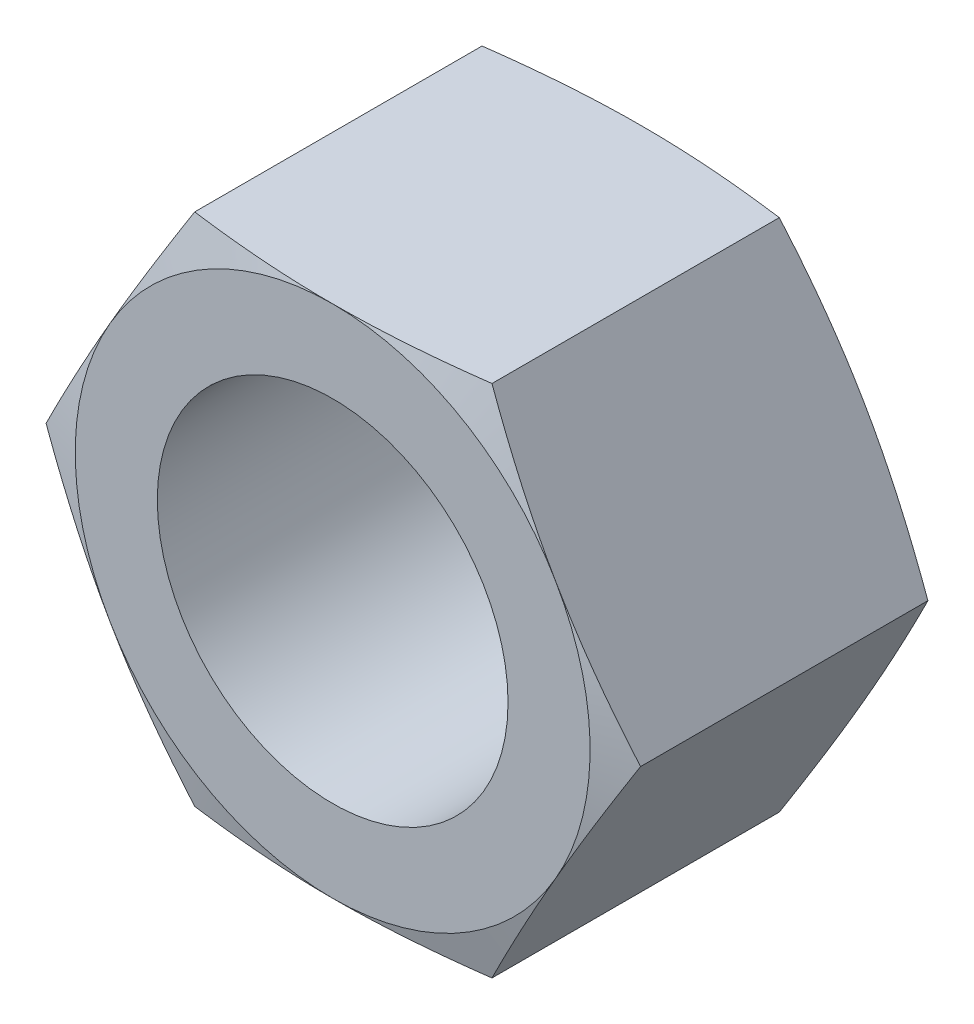
from build123d import *

# Parameters (mm, degrees)
SKETCH1_R          = 15
BASE_EXTRUDE_DEPTH = 26.4
SKETCH2_OUTSIDE_W  = 350.938
SKETCH2_OUTSIDE_H  = 344.126
SKETCH2_OUTSIDE_R  = 22.018695891
CUT_EXTRUDE1_DEPTH = 38
CUT_EXTRUDE1_DRAFT = -75
SKETCH3_OUTSIDE_W  = 350.938
SKETCH3_OUTSIDE_H  = 344.126
SKETCH3_OUTSIDE_R  = 22.018695891
CUT_EXTRUDE2_DEPTH = 38
CUT_EXTRUDE2_DRAFT = -75


with BuildPart() as part:
    # Sketch1 → Base-Extrude (new body)
    with BuildSketch(Plane.XY):
        Polygon((12.7125, 22.018695891), (-12.7125, 22.018695891), (-25.425, 0), (-12.7125, -22.018695891), (12.7125, -22.018695891), (25.425, 0), align=None)
        Circle(SKETCH1_R, mode=Mode.SUBTRACT)
    extrude(amount=BASE_EXTRUDE_DEPTH)


with BuildPart() as cut_extrude1_tool:
    # Sketch2 outside → Cut-Extrude1 (with draft: the straight prism first)
    with BuildSketch(Plane(origin=(0, 0, 0), x_dir=(-1, 0, 0), z_dir=(0, 0, -1))):
        Rectangle(SKETCH2_OUTSIDE_W, SKETCH2_OUTSIDE_H)
        Circle(SKETCH2_OUTSIDE_R, mode=Mode.SUBTRACT)
    extrude(amount=-CUT_EXTRUDE1_DEPTH)
    # Cut-Extrude1: the draft: its side faces are tilted about the plane it starts from
    cut_extrude1_sides = [cut_extrude1_tool.faces().sort_by_distance(p)[0] for p in [
        (0, -172.063, 19),
        (-175.469, 0, 19),
        (0, 172.063, 19),
        (175.469, 0, 19),
        (22.018695891, 0, 19),
    ]]
    draft(cut_extrude1_sides, Plane(origin=(0, 0, 0), x_dir=(-1, 0, 0), z_dir=(0, 0, -1)), CUT_EXTRUDE1_DRAFT)


with BuildPart() as part_1:
    add(part.part)

    # Cut-Extrude1: cut by cut_extrude1_tool
    add(cut_extrude1_tool.part, mode=Mode.SUBTRACT)


with BuildPart() as cut_extrude2_tool:
    # Sketch3 outside → Cut-Extrude2 (with draft: the straight prism first)
    with BuildSketch(Plane.XY.offset(26.4)):
        Rectangle(SKETCH3_OUTSIDE_W, SKETCH3_OUTSIDE_H)
        Circle(SKETCH3_OUTSIDE_R, mode=Mode.SUBTRACT)
    extrude(amount=-CUT_EXTRUDE2_DEPTH)
    # Cut-Extrude2: the draft: its side faces are tilted about the plane it starts from
    cut_extrude2_sides = [cut_extrude2_tool.faces().sort_by_distance(p)[0] for p in [
        (0, -172.063, 7.4),
        (175.469, 0, 7.4),
        (0, 172.063, 7.4),
        (-175.469, 0, 7.4),
        (-22.018695891, 0, 7.4),
    ]]
    draft(cut_extrude2_sides, Plane.XY.offset(26.4), CUT_EXTRUDE2_DRAFT)


with BuildPart() as part_2:
    add(part_1.part)

    # Cut-Extrude2: cut by cut_extrude2_tool
    add(cut_extrude2_tool.part, mode=Mode.SUBTRACT)


solid = part_2.part
